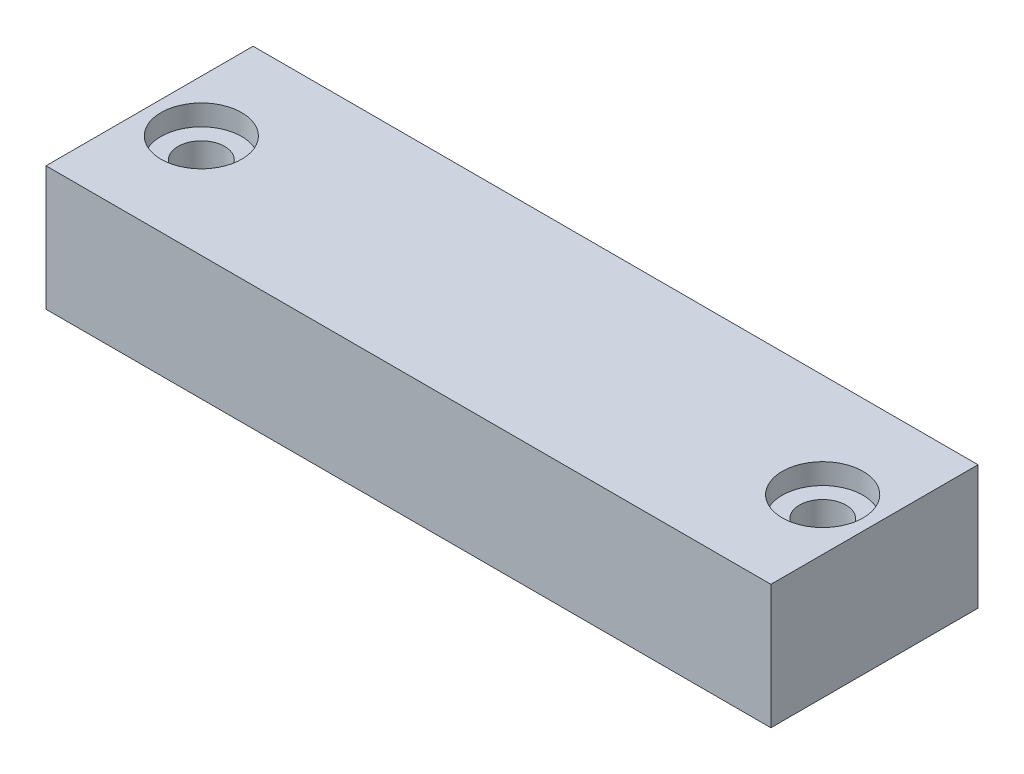
from build123d import *

# Parameters (mm, degrees)
SKETCH_1_W                = 70
SKETCH_1_H                = 20
EXTRUDE_1_DEPTH           = 12
HOLE_WIZARD_1_D           = 4.5
HOLE_WIZARD_1_CBORE_D     = 7.8
HOLE_WIZARD_1_CBORE_DEPTH = 2


with BuildPart() as part:
    # 草图1 → 凸台-拉伸1 (new body)
    with BuildSketch(Plane(origin=(0, 0, 0), x_dir=(1, 0, 0), z_dir=(0, 1, 0))):
        Rectangle(SKETCH_1_W, SKETCH_1_H)
    extrude(amount=EXTRUDE_1_DEPTH)

    # 打孔尺寸(%根据)内六角圆柱头螺钉的类型1 (through all)
    with Locations(Plane(origin=(0, 12, 0), x_dir=(1, 0, 0), z_dir=(0, 1, 0))):
        with Locations((-30, 0), (30, 0)):
            CounterBoreHole(HOLE_WIZARD_1_D / 2, HOLE_WIZARD_1_CBORE_D / 2, HOLE_WIZARD_1_CBORE_DEPTH)


solid = part.part
